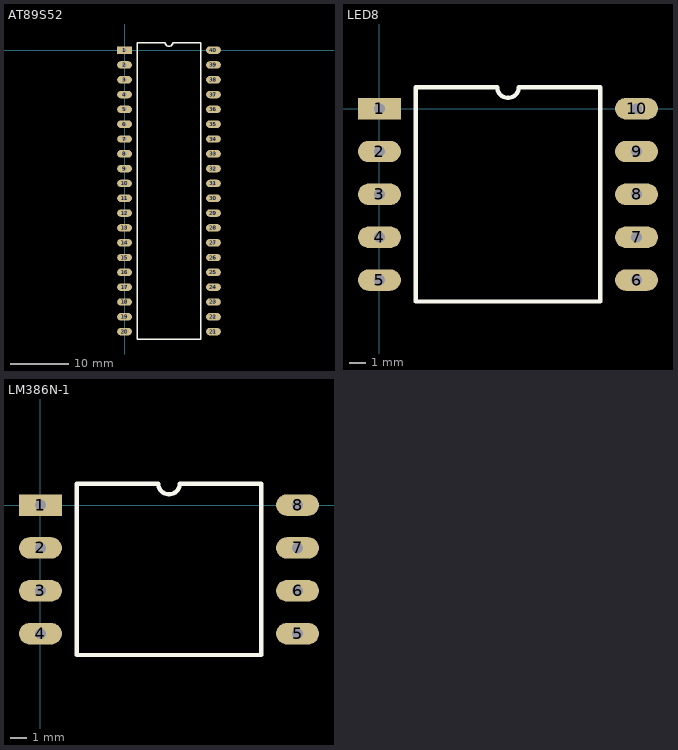
[diagram p0: the footprints below, top view; thin cyan lines are the x and y axes]
# Altium footprint library MISC82805-4.PcbLib: 3 footprints
Each footprint in its own frame and in the unit in brackets; x right, y up, seen from the top. Pads: shape width x height; smd on the part's side, far side on the other; paste and mask are expansions set on the pad; w line width, h text height; cw(c..) or ccw(c..) is an arc to the next point about the centre after c.

## AT89S52 [mil]
pads (40):
  rect 100x50 hole 25: 1(0,0)
  oval 100x50 hole 25: 2(0,-100) 3(0,-200) 4(0,-300) 5(0,-400) 6(0,-500) 7(0,-600) 8(0,-700) 9(0,-800) 10(0,-900) 11(0,-1000) 12(0,-1100) 13(0,-1200) 14(0,-1300) 15(0,-1400) 16(0,-1500) 17(0,-1600) 18(0,-1700) 19(0,-1800) 20(0,-1900) 21(600,-1900) 22(600,-1800) 23(600,-1700) 24(600,-1600) 25(600,-1500) 26(600,-1400) 27(600,-1300) 28(600,-1200) 29(600,-1100) 30(600,-1000) 31(600,-900) 32(600,-800) 33(600,-700) 34(600,-600) 35(600,-500) 36(600,-400) 37(600,-300) 38(600,-200) 39(600,-100) 40(600,0)
Top Overlay:
  lines w10: 85,-1950 85,50 275,50 ccw(c300,50) 325,50 515,50 515,-1950 85,-1950

## LED8 [mil]
pads (10):
  rect 100x50 hole 25: 1(0,0)
  oval 100x50 hole 25: 2(0,-100) 3(0,-200) 4(0,-300) 5(0,-400) 6(600,-400) 7(600,-300) 8(600,-200) 9(600,-100) 10(600,0)
Top Overlay:
  lines w10: 85,-450 85,50 275,50 ccw(c300,50) 325,50 515,50 515,-450 85,-450

## LM386N-1 [mil]
pads (8):
  rect 100x50 hole 25: 1(0,0)
  oval 100x50 hole 25: 2(0,-100) 3(0,-200) 4(0,-300) 5(600,-300) 6(600,-200) 7(600,-100) 8(600,0)
Top Overlay:
  lines w10: 85,-350 85,50 275,50 ccw(c300,50) 325,50 515,50 515,-350 85,-350